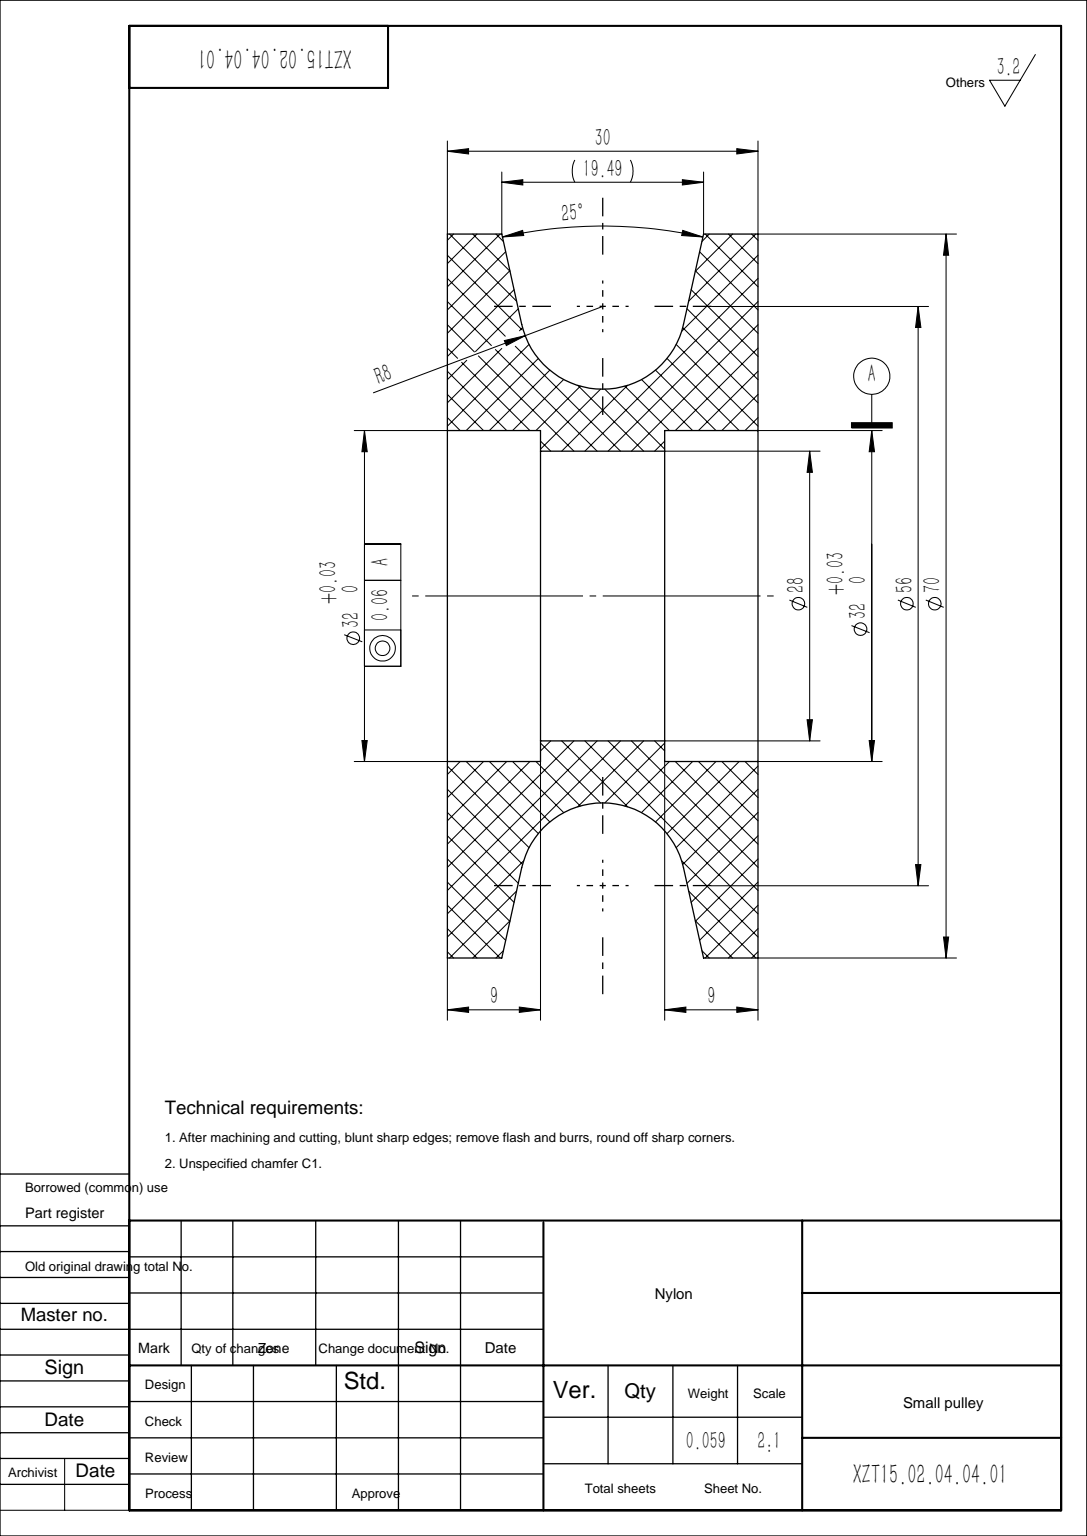
from build123d import *


with BuildPart() as part:
    # Sketch1 → Revolve1 (revolve)
    with BuildSketch(Plane.XY, mode=Mode.PRIVATE) as revolve1_sk:
        with BuildLine():
            Line((-6, 14), (6, 14))
            Line((6, 14), (6, 16))
            Line((6, 16), (15, 16))
            Line((15, 16), (15, 35))
            Line((15, 35), (9.746098753, 35))
            Line((9.746098753, 35), (7.810368057, 26.268483088))
            ThreePointArc((7.810368057, 26.268483088), (5.007387777, 21.760924135), (0, 20))
            ThreePointArc((0, 20), (-5.007387777, 21.760924135), (-7.810368057, 26.268483088))
            Line((-7.810368057, 26.268483088), (-9.746098753, 35))
            Line((-9.746098753, 35), (-15, 35))
            Line((-15, 35), (-15, 16))
            Line((-15, 16), (-6, 16))
            Line((-6, 16), (-6, 14))
        make_face()
    revolve(revolve1_sk.sketch.rotate(Axis((0, 0, 0), (1, 0, 0)), 90), axis=Axis((0, 0, 0), (1, 0, 0)))


solid = part.part
